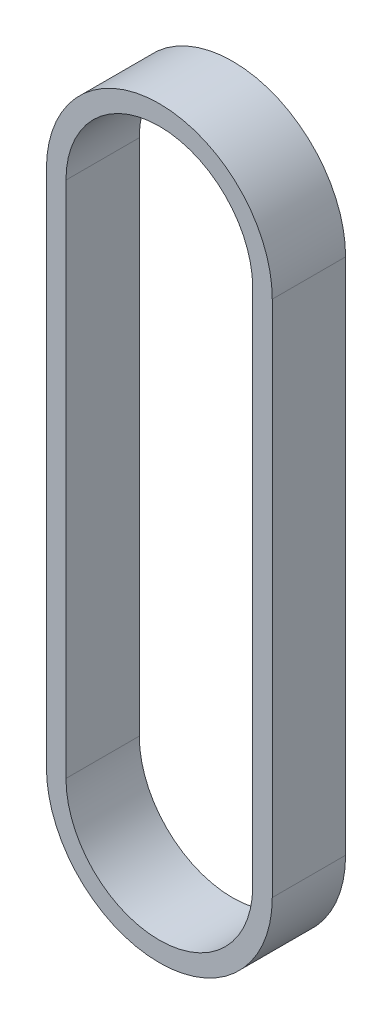
from build123d import *

# Parameters (mm, degrees)
EXTRUDE_1_DEPTH = 7.5


with BuildPart() as part:
    # 草图2 → 拉伸-薄壁1 (new, symmetric)
    with BuildSketch(Plane.XY):
        with BuildLine():
            Line((23.1, 106), (23.1, 0))
            ThreePointArc((23.1, 0), (0, -23.1), (-23.1, 0))
            Line((-23.1, 0), (-23.1, 106))
            ThreePointArc((-23.1, 106), (0, 129.1), (23.1, 106))
        make_face()
        with BuildLine():
            Line((19.1, 106), (19.1, 0))
            ThreePointArc((19.1, 0), (0, -19.1), (-19.1, 0))
            Line((-19.1, 0), (-19.1, 106))
            ThreePointArc((-19.1, 106), (0, 125.1), (19.1, 106))
        make_face(mode=Mode.SUBTRACT)
    extrude(amount=EXTRUDE_1_DEPTH, both=True)


solid = part.part
